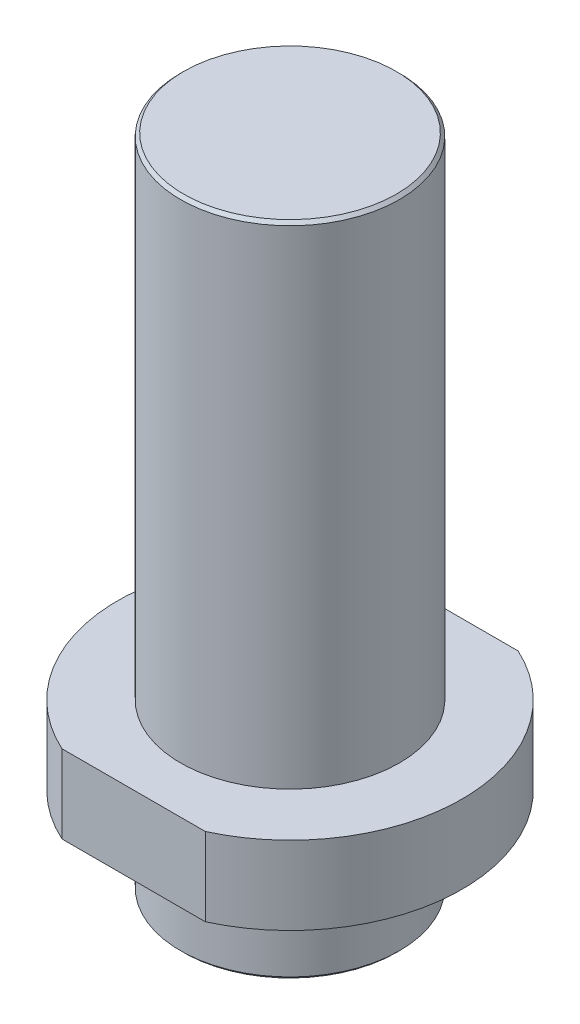
from build123d import *

# Parameters (mm, degrees)
CUT_EXTRUDE1_DEPTH = 176.211301005


with BuildPart() as part:
    # Sketch1 → Revolve1 (revolve)
    with BuildSketch(Plane.XY):
        Polygon((0, 0), (-34, 0), (-35, 1), (-35, 28), (-55, 28), (-55, 53), (-35, 53), (-35, 209), (-34, 210), (0, 210), align=None)
    revolve(axis=Axis((0, 210, 0), (0, -1, 0)))

    # Sketch2 → Cut-Extrude1 (cut, through all)
    with BuildSketch(Plane(origin=(0, 53, 0), x_dir=(1, 0, 0), z_dir=(0, 1, 0))):
        with BuildLine():
            Line((-22.912878475, 50), (22.912878475, 50))
            ThreePointArc((22.912878475, 50), (0, 55), (-22.912878475, 50))
        make_face()
        with BuildLine():
            Line((-22.912878475, -50), (22.912878475, -50))
            ThreePointArc((22.912878475, -50), (0, -55), (-22.912878475, -50))
        make_face()
    extrude(amount=-CUT_EXTRUDE1_DEPTH, mode=Mode.SUBTRACT)


solid = part.part
